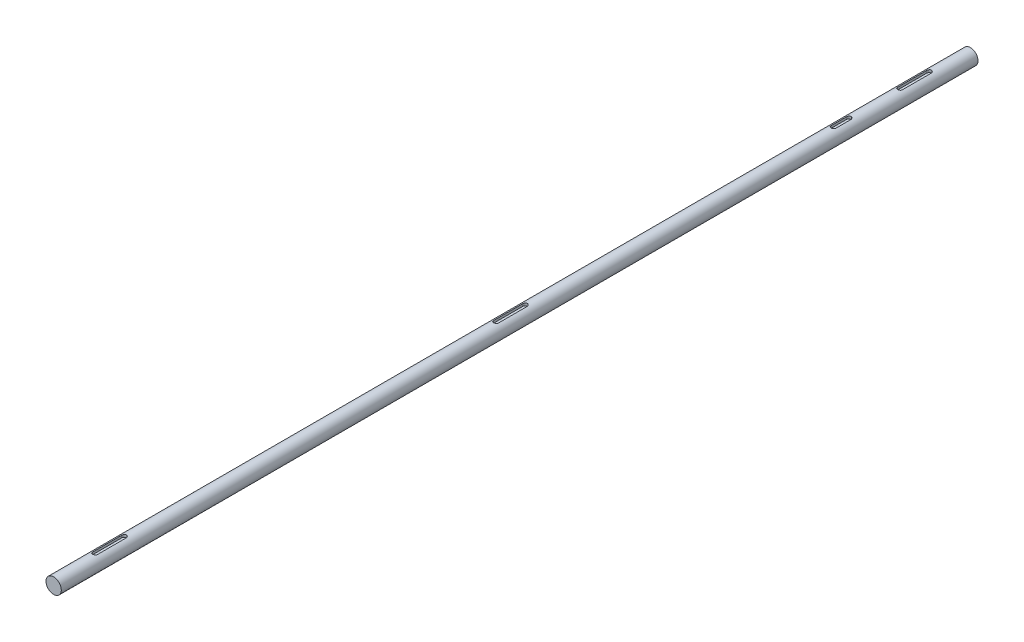
SolidWorks part; units mm, degrees
ref_plane "前视基准面" through (0, 0, 0) normal (0, 0, 1) x (1, 0, 0)
ref_plane "上视基准面" through (0, 0, 0) normal (0, 1, 0) x (1, 0, 0)
ref_plane "右视基准面" through (0, 0, 0) normal (1, 0, 0) x (0, 0, -1)
sketch "草图1" plane through (0, 0, 0) normal (0, 0, 1) x (1, 0, 0)
  circle A0 centre (0, 0) radius 10
  dimension "D1" = 20
extrude "凸台-拉伸1" add sketch "草图1" along normal mid plane 1198
sketch "草图3" plane through (0, 0, 0) normal (0, 1, 0) x (1, 0, 0)
  line L0 (0, 545) -> (0, 507) construction
  line L1 (0, 507) -> (0, 440) construction
  line L2 (0, 507) -> (0, 545) construction
  line L3 (-3, 507) -> (-3, 545)
  line L4 (3, 507) -> (3, 545)
  line L5 (0, 0) -> (127.8063, 0) construction
  line L6 (0, -545) -> (0, -507) construction
  line L7 (0, -507) -> (0, -545) construction
  line L8 (-3, -507) -> (-3, -545)
  line L9 (3, -507) -> (3, -545)
  line L11 (0, 440) -> (0, 420) construction
  line L12 (3, 440) -> (3, 420)
  line L13 (-3, 440) -> (-3, 420)
  line L15 (10, 599) -> (-10, 599) construction
  line L16 (0, 17) -> (0, -21) construction
  line L17 (0, -21) -> (0, 17) construction
  line L18 (-3, -21) -> (-3, 17)
  line L19 (3, -21) -> (3, 17)
  arc A0 (-3, 507) -> (3, 507) centre (0, 507) ccw
  arc A1 (3, 545) -> (-3, 545) centre (0, 545) ccw
  arc A2 (-3, -507) -> (3, -507) centre (0, -507) cw
  arc A3 (3, -545) -> (-3, -545) centre (0, -545) cw
  arc A4 (3, 440) -> (-3, 440) centre (0, 440) ccw
  arc A5 (-3, 420) -> (3, 420) centre (0, 420) ccw
  arc A6 (-3, -21) -> (3, -21) centre (0, -21) ccw
  arc A7 (3, 17) -> (-3, 17) centre (0, 17) ccw
  point P5 (0, 526)
  point P14 (0, -526)
  point P19 (0, 430)
  point P31 (0, -2)
  dimension "D1" = 6
  dimension "D2" = 54
  dimension "D3" = 38
  dimension "D4" = 20
  dimension "D5" = 67
  dimension "D6" = 2
extrude "切除-拉伸3" cut sketch "草图3" against normal blind 3.5 from offset 10
